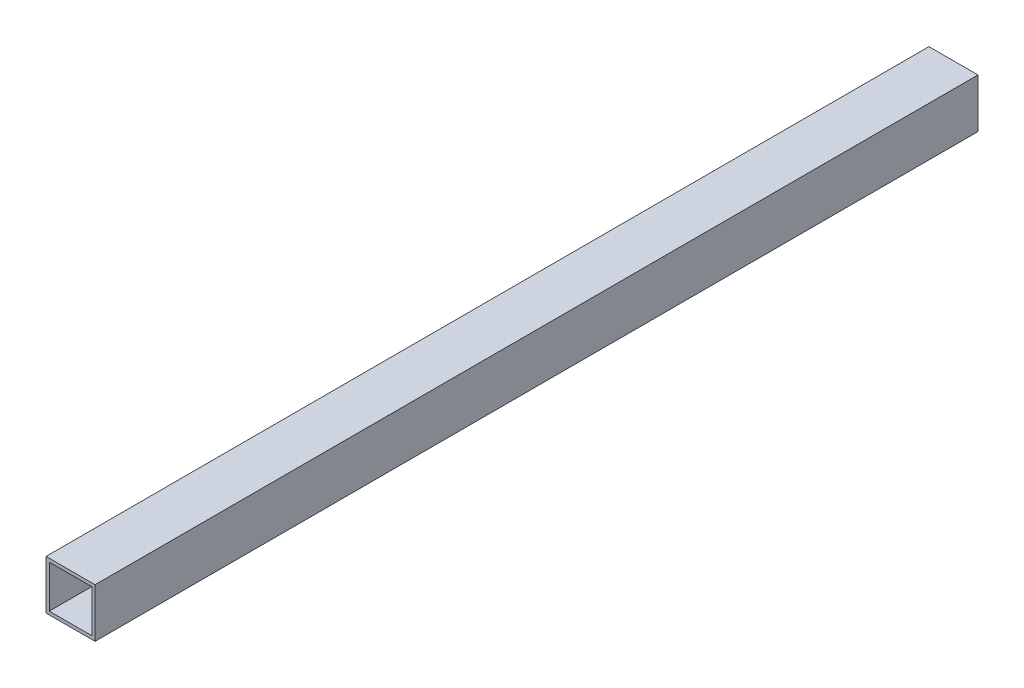
from build123d import *

# Parameters (mm, degrees)
SKETCH_1_W      = 30
SKETCH_1_H      = 30
SKETCH_1_W_2    = 26
SKETCH_1_H_2    = 26
EXTRUDE_1_DEPTH = 270


with BuildPart() as part:
    # 草图1 → 凸台-拉伸1 (new, symmetric)
    with BuildSketch(Plane.XY):
        Rectangle(SKETCH_1_W, SKETCH_1_H)
        Rectangle(SKETCH_1_W_2, SKETCH_1_H_2, mode=Mode.SUBTRACT)
    extrude(amount=EXTRUDE_1_DEPTH, both=True)


solid = part.part
